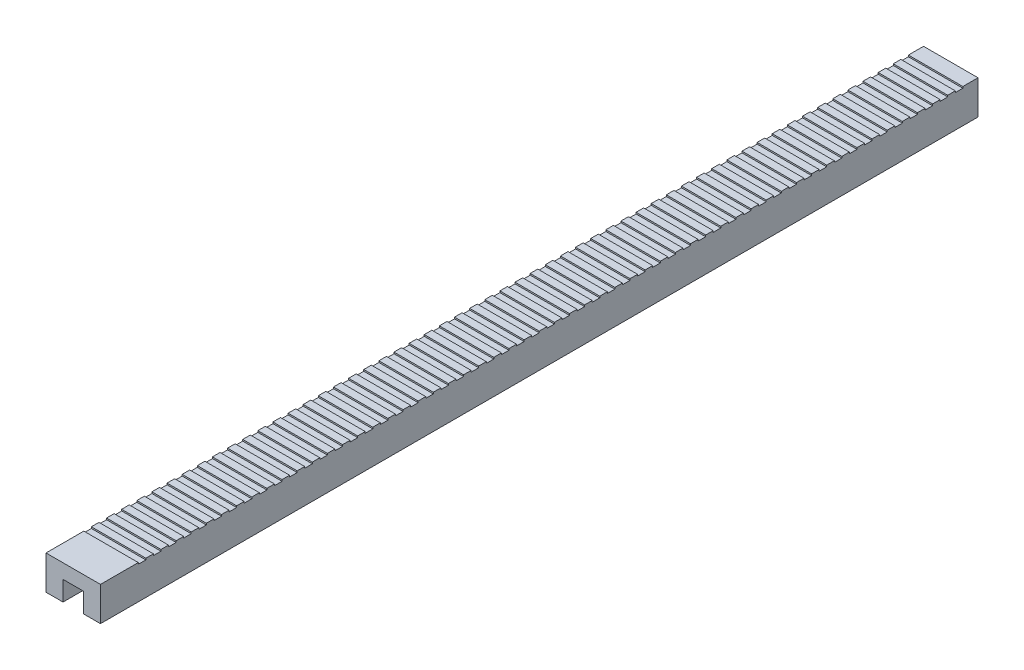
from build123d import *

# Parameters (mm, degrees)
BOSS_EXTRUDE1_DEPTH = 1160
SKETCH2_W           = 72
SKETCH2_H           = 10
CUT_EXTRUDE1_DEPTH  = 2
LPATTERN1_COUNT     = 55
LPATTERN1_PITCH     = 20


with BuildPart() as part:
    # Sketch1 → Boss-Extrude1 (new body)
    with BuildSketch(Plane.XY):
        Polygon((0, 3.5), (0, 22.5), (-36, 22.5), (-36, -22.5), (-13.5, -22.5), (-13.5, 3.5), align=None)
        Polygon((36, 22.5), (0, 22.5), (0, 3.5), (13.5, 3.5), (13.5, -22.5), (36, -22.5), align=None)
    extrude(amount=BOSS_EXTRUDE1_DEPTH)

    # Sketch2 → Cut-Extrude1 (cut)
    with BuildSketch(Plane(origin=(0, 22.5, 0), x_dir=(1, 0, 0), z_dir=(0, 1, 0))):
        with Locations((0, -25)):
            Rectangle(SKETCH2_W, SKETCH2_H)
    cut_extrude1 = extrude(amount=-CUT_EXTRUDE1_DEPTH, mode=Mode.SUBTRACT)

    # LPattern1: Cut-Extrude1 ×55
    with Locations(*[(0, 0, i * LPATTERN1_PITCH) for i in range(1, LPATTERN1_COUNT)]):
        add(cut_extrude1, mode=Mode.SUBTRACT)


solid = part.part
